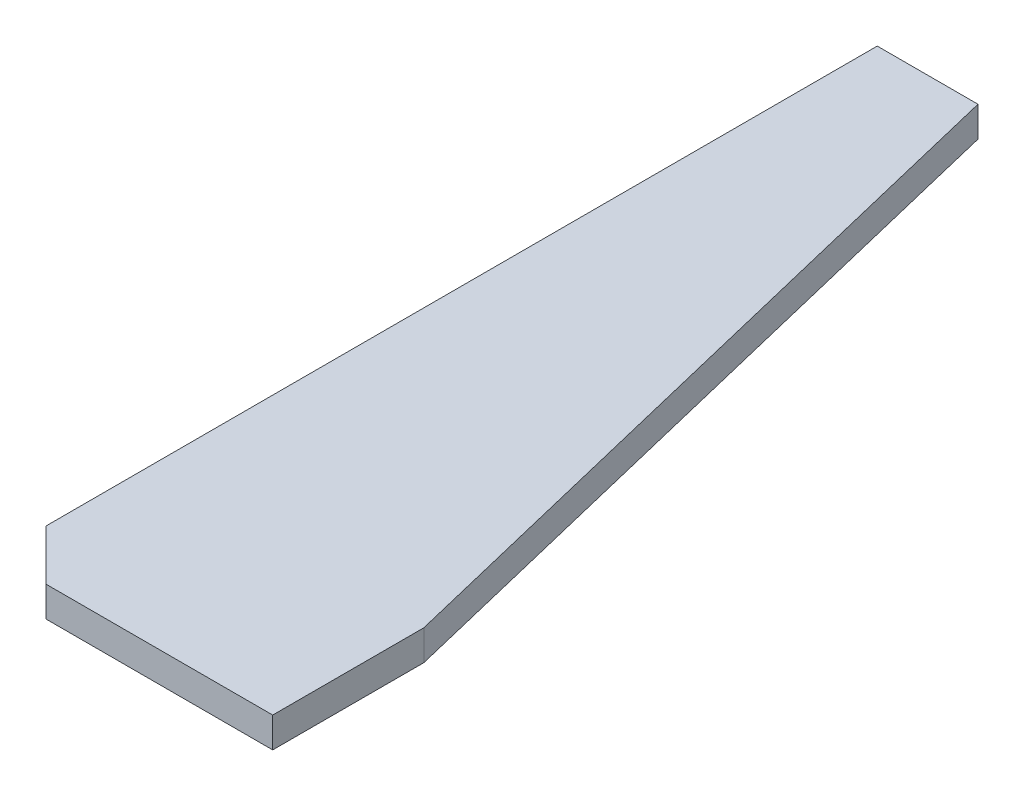
SolidWorks part; units mm, degrees
material "Q235B"
ref_plane "Front Plane" through (0, 0, 0) normal (0, 0, 1) x (1, 0, 0)
ref_plane "Top Plane" through (0, 0, 0) normal (0, 1, 0) x (1, 0, 0)
ref_plane "Right Plane" through (0, 0, 0) normal (1, 0, 0) x (0, 0, -1)
sketch "Sketch1" plane through (0, 0, 0) normal (0, 1, 0) x (1, 0, 0)
  line L10 (0, 0) -> (-20, 20) construction
  line L11 (-20, 20) -> (-20, 350)
  line L13 (-20, 350) -> (20, 350)
  line L14 (20, 350) -> (90, 60)
  line L15 (90, 60) -> (90, 0)
  line L16 (90, 0) -> (0, 0)
  line L17 (-20, 20) -> (-20, 0)
  line L18 (-20, 0) -> (0, 0)
  dimension "D1" = 20
  dimension "D5" = 60
  dimension "D8" = 40
  dimension "D2" = 20
  dimension "D4" = 110
  dimension "D7" = 350
extrude "Boss-Extrude1" add sketch "Sketch1" along normal mid plane 12
chamfer "Chamfer1" distance 20 angle 45 1 edges at (-20, 0, 0)
